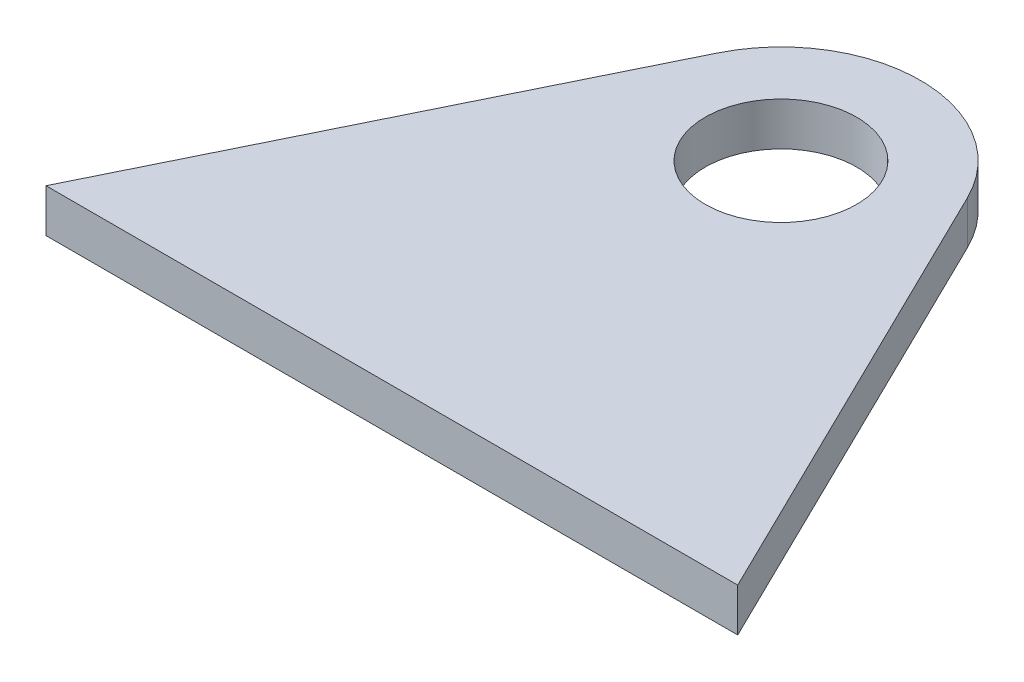
from build123d import *

# Parameters (mm, degrees)
SKETCH_1_R          = 17.25
EXTRUDE_1_DEPTH     = 10
SKETCH_2_R          = 17.5
CUT_EXTRUDE_1_DEPTH = 10


with BuildPart() as part:
    # 草图1 → 凸台-拉伸1 (new body)
    with BuildSketch(Plane(origin=(0, 0, 0), x_dir=(1, 0, 0), z_dir=(0, 1, 0))):
        with BuildLine():
            Line((0, 0), (160, 0))
            Line((160, 0), (108.961672936, 104.187459277))
            ThreePointArc((108.961672936, 104.187459277), (80, 122.25), (51.038327064, 104.187459277))
            Line((51.038327064, 104.187459277), (0, 0))
        make_face()
        with Locations(Location((80, 90, 0), (0, 0, 270))):
            Circle(SKETCH_1_R, mode=Mode.SUBTRACT)
    extrude(amount=EXTRUDE_1_DEPTH)

    # 草图2 → 切除-拉伸1 (cut)
    with BuildSketch(Plane(origin=(0, 10, 0), x_dir=(1, 0, 0), z_dir=(0, 1, 0))):
        with Locations(Location((80, 90, 0), (0, 0, 270))):
            Circle(SKETCH_2_R)
    extrude(amount=-CUT_EXTRUDE_1_DEPTH, mode=Mode.SUBTRACT)


solid = part.part
